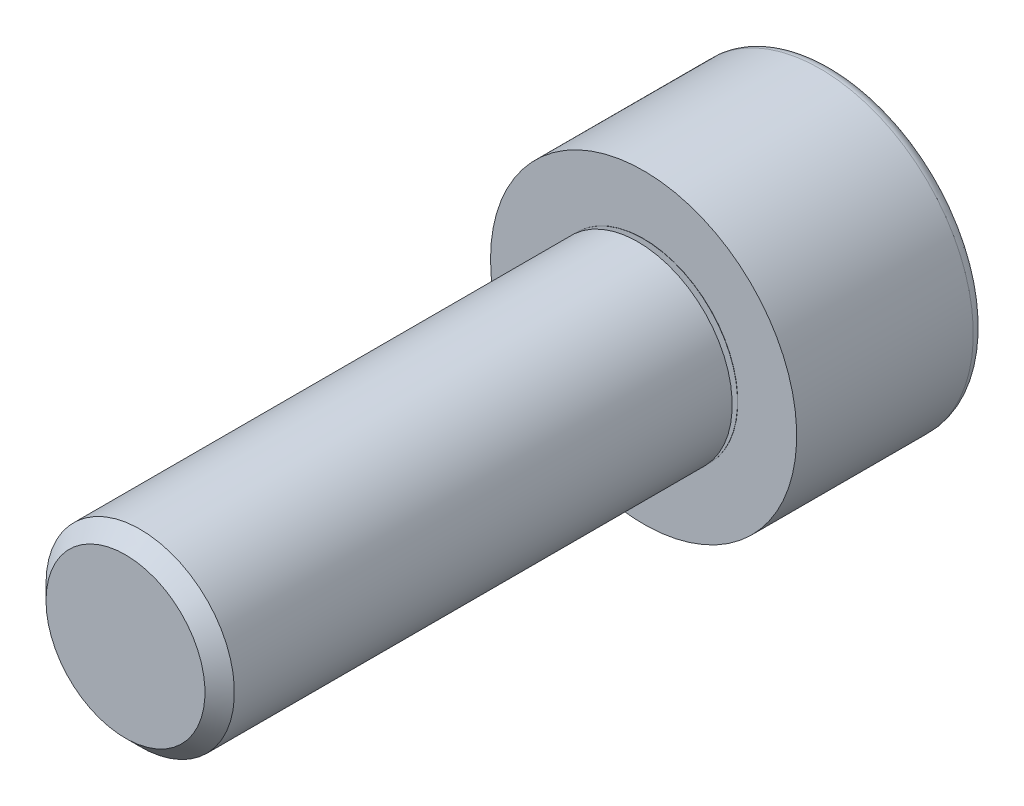
SolidWorks part; units mm, degrees
ref_plane "Front" through (0, 0, 0) normal (0, 0, 1) x (1, 0, 0)
ref_plane "Top" through (0, 0, 0) normal (0, 1, 0) x (1, 0, 0)
ref_plane "Right" through (0, 0, 0) normal (1, 0, 0) x (0, 0, -1)
sketch "Logo3_Revol_Axis" plane through (0, 0, 0) normal (0, 1, 0) x (1, 0, 0)
  line L0 (0, -43.5172) -> (0, 43.5172) construction
sketch "Logo3_bib1" plane through (0, 0, 0) normal (0, -1, 0) x (-1, 0, 0)
  line L0 (0, -22) -> (0, 8)
  line L1 (0, 8) -> (6, 8)
  line L2 (6.5, 7.5) -> (6.5, 0)
  line L3 (6.5, 0) -> (4, 0)
  line L4 (4, 0) -> (4, -0.01)
  line L5 (4, -21.375) -> (3.375, -22)
  line L6 (3.375, -22) -> (0, -22)
  line L7 (4, -0.01) -> (3.4884, -0.01)
  line L8 (3.4816, -0.0488) -> (4, -0.2375)
  line L9 (4, -0.2375) -> (4, -21.375)
  line L10 (0, 10.5852) -> (0, -63.2873) construction
  arc A0 (6, 8) -> (6.5, 7.5) centre (6, 7.5) cw
  arc A1 (3.4884, -0.01) -> (3.4816, -0.0488) centre (3.4884, -0.03) ccw
  point P17 (3.375, -0.01)
revolve "Revolve1" add sketch "Logo3_bib1" angle 360 about L10
cosmetic thread "Cosmetic Thread1" parameters "D2"=6.75
sketch "Logo3_bib2" plane through (0, 0, -8) normal (0, 0, -1) x (1, 0, 0)
  line L1 (3.4641, 0) -> (1.7321, 3)
  line L2 (1.7321, 3) -> (-1.7321, 3)
  line L3 (-1.7321, 3) -> (-3.4641, 0)
  line L4 (-3.4641, 0) -> (-1.7321, -3)
  line L5 (-1.7321, -3) -> (1.7321, -3)
  line L6 (1.7321, -3) -> (3.4641, 0)
  circle A0 centre (0, 0) radius 3 construction
extrude "Cut-Extrude1" cut sketch "Logo3_bib2" against normal blind 3
equation "\"DIA2@XZQB7_bib1\" = \"XZQB7_d1-pas@XZQB7_bib1\""
equation "\"LGT1@XZQB7_bib1\" = \"XZQB7_d1@XZQB7_bib1\""
equation "\"D1@Cut-Extrude1\" = \"XZQB7_c1@XZQB7_bib2\"/2."
equation "\"D2@Cosmetic Thread1\" = \"XZQB7_d1-pas@XZQB7_bib1\""
